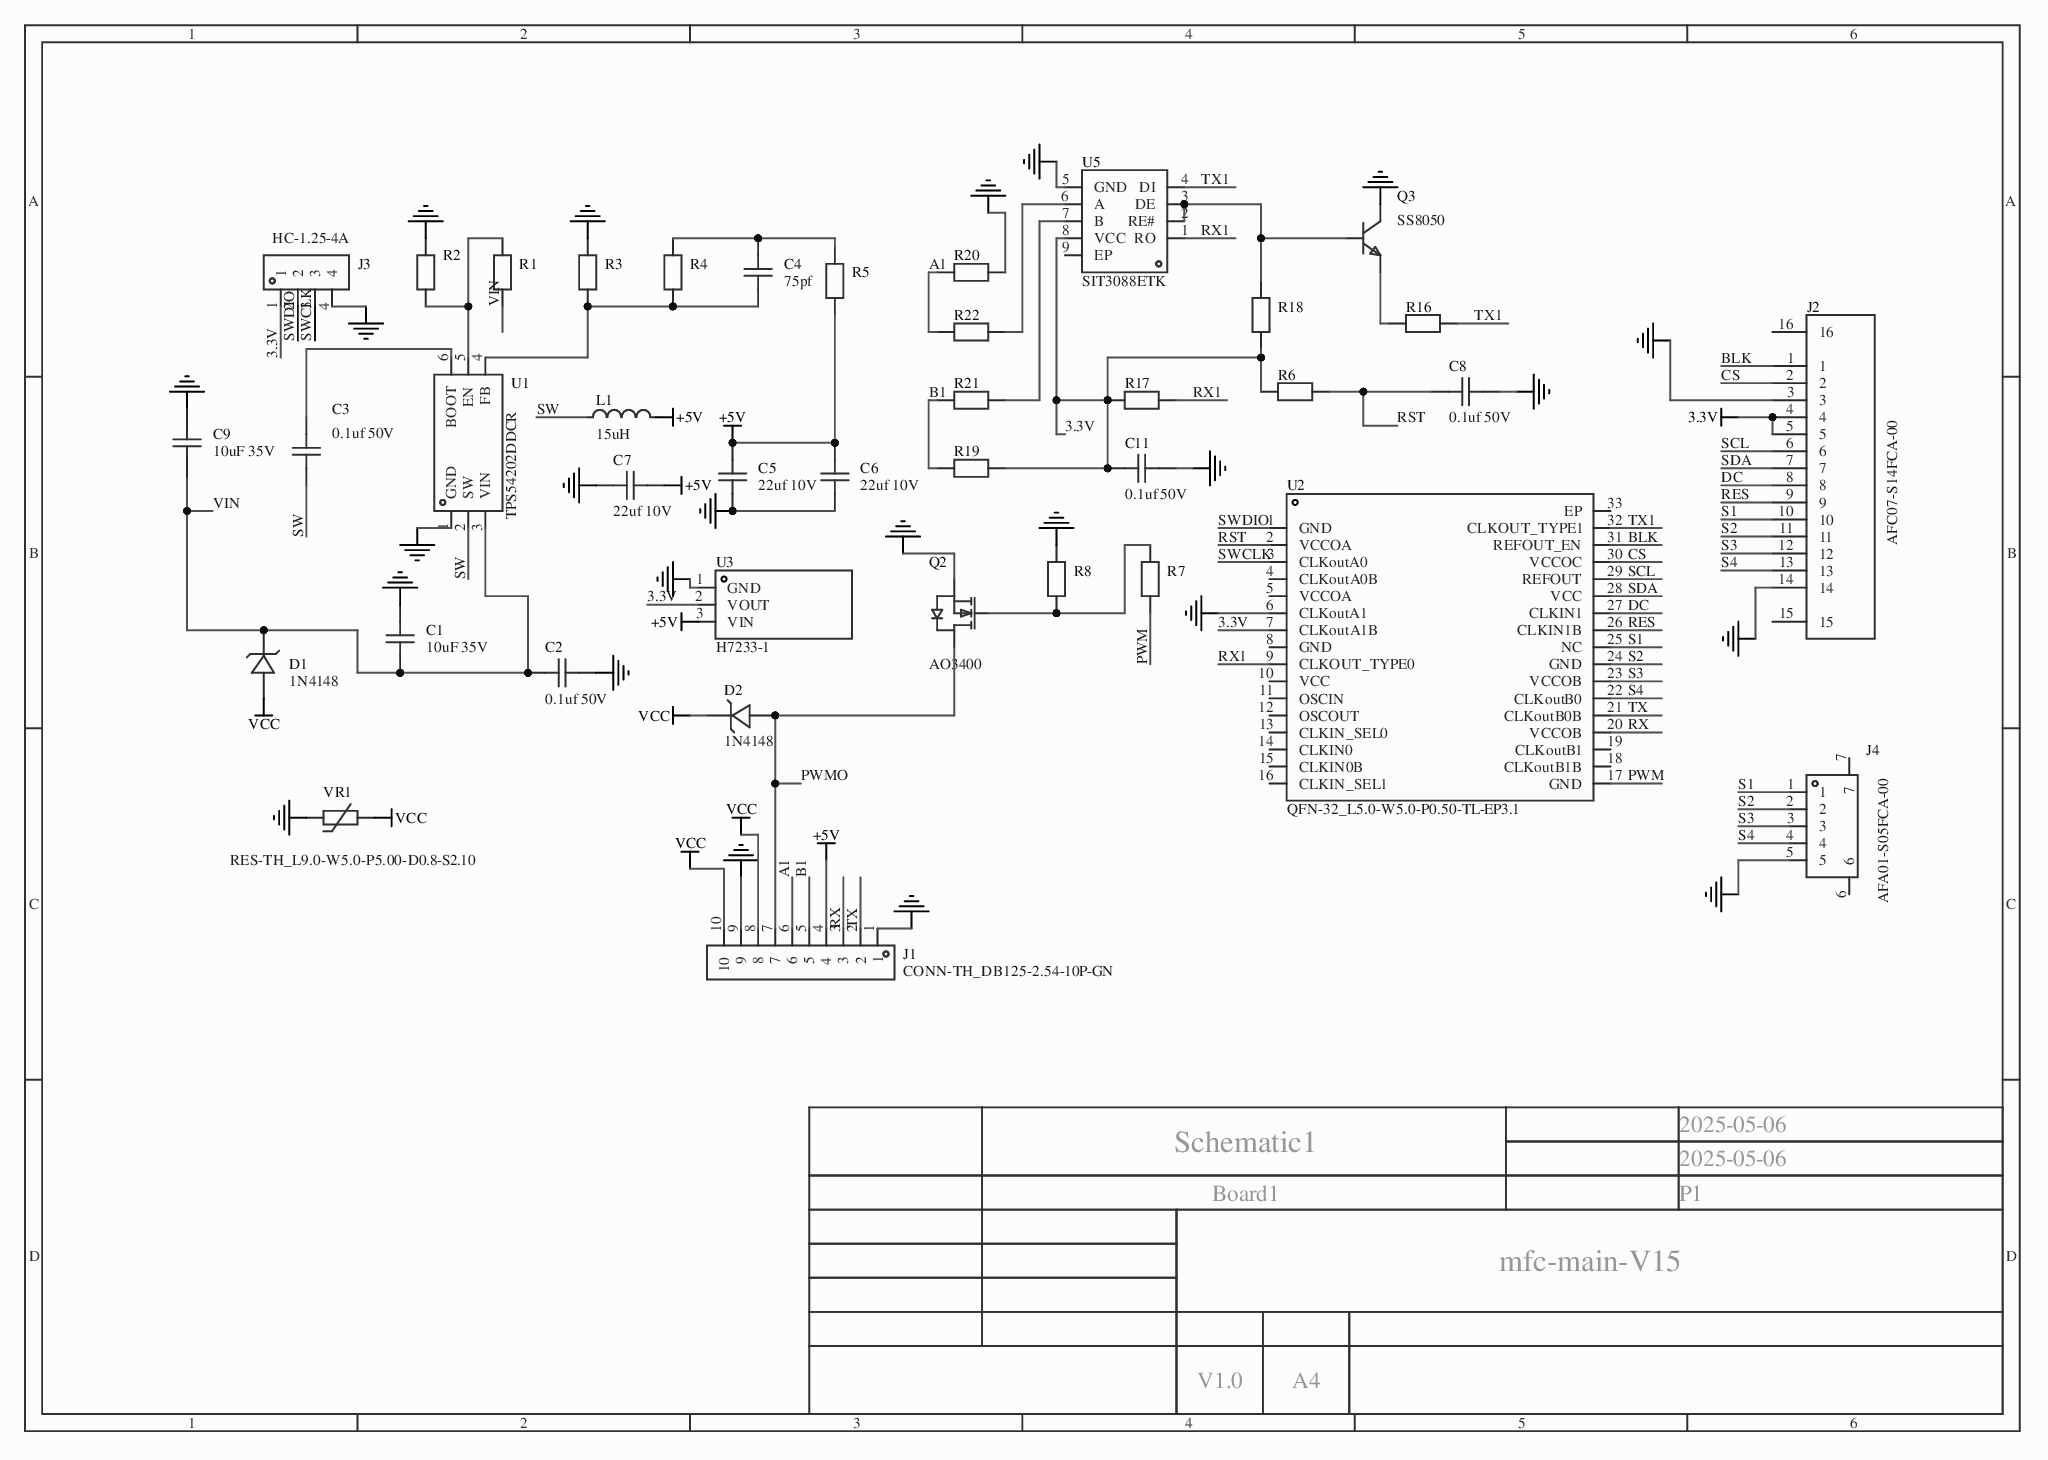
[diagram p0: MISC84392-2.SchDoc]
# Altium project MISC84392-4.PrjPcb
1 sheet, 39 parts. Net scope: global (net labels, ports and power ports of the same name join across sheets).
Board file: MISC84392.PcbDoc

## Sheet MISC84392-2.SchDoc
size 307 x 218 mm; Symbol: Drawing-Symbol_A4; Device: Drawing-Symbol_A4; Version: V1.0; Page Size: A4; @Project Name: mfc-main-V15; @Page Count: 1; @Update Date: 2025-05-06; @Create Date: 2025-05-06; @Schematic Name: Schematic1; @Page No: 1; @Page Name: P1; @Create Time: 07:06:31; @Update Time: 15:06:31; Width: 1170; Height: 825; Region Start: 1; X Region Count: 6; Y Region Count: 4; Blade Width: 10; Title Block Position: 3; @Board Name: Board1

### Parts
C1  10uF 35V  [C0805]
C2  0.1uf 50V  [C0603]
C3  0.1uf 50V  [C0603]
C4  75pf  [C0603]
C5  22uf 10V  [C0603]
C6  22uf 10V  [C0603]
C7  22uf 10V  [C0603]
C8  0.1uf 50V  [C0603]
C9  10uF 35V  [C0805]
C11  0.1uf 50V  [C0603]
D1  1N4148  [SOD-123_L2.7-W1.7-LS3.8-RD]
D2  1N4148  [SOD-123_L2.7-W1.7-LS3.8-RD]
J1  CONN-TH_DB125-2.54-10P-GN  [CONN-TH_DB125-2.54-10P-GN]
J2  AFC07-S14FCA-00  [FPC-SMD_14P-P0.50_AFC07-S14FCA-00]
J3  HC-1.25-4A  [CONN-TH_4P-P1.25_HCTL_HC-1.25-4A]
J4  AFA01-S05FCA-00  [FPC-SMD_AFA01-S05FCA-00]
L1  15uH  [IND-SMD_L3.5-W3.0]
Q2  AO3400  [SOT-23-3_L2.9-W1.3-P1.90-LS2.4-BL-2]
Q3  SS8050  [SOT-23-3_L2.9-W1.3-P1.90-LS2.4-BR]
R1  (no value)  [R0603]
R2  (no value)  [R0603]
R3  (no value)  [R0603]
R4  (no value)  [R0603]
R5  (no value)  [R0603]
R6  (no value)  [R0603]
R7  (no value)  [R0603]
R8  (no value)  [R0603]
R16  (no value)  [R0603]
R17  (no value)  [R0603]
R18  (no value)  [R0603]
R19  (no value)  [R0603]
R20  (no value)  [R0603]
R21  (no value)  [R0603]
R22  (no value)  [R0603]
U1  TPS54202DDCR  [SOT-23-6_L2.9-W1.6-P0.95-LS2.8-BL]
U2  QFN-32_L5.0-W5.0-P0.50-TL-EP3.1  [QFN-32_L5.0-W5.0-P0.50-TL-EP3.1]
U3  H7233-1  [SOT-23-3_L2.9-W1.3-P1.90-LS2.4-BR]
U5  SIT3088ETK  [DFN-8_L3.0-W3.0-P0.65-BL-EP]
VR1  RES-TH_L9.0-W5.0-P5.00-D0.8-S2.10  [RES-TH_L9.0-W5.0-P5.00-D0.8-S2.10]

### Nets
3.3V: C11.2 J2.4 J2.5 J3.1 R6.1 R17.1 R18.1 R19.2 U2.7(CLKoutA1B) U3.2(VOUT) U5.8(VCC)
+5V: C5.1 C6.1 C7.1 J1.4 L1.2 R5.1 U3.3(VIN)
GND: C1.2 C2.1 C5.2 C6.2 C7.2 C8.1 C9.2 C11.1 J1.1 J1.9 J2.3 J2.14 J3.4 J4.5 Q2.2(S) Q3.3(C) R2.2 R3.2 R8.2 R20.2 U1.1(GND) U2.6(CLKoutA1) U3.1(GND) U5.5(GND) VR1.1
VCC: D1.2(A) D2.1(K) J1.8 J1.10 VR1.2
A1: J1.6 R20.1 R22.1
B1: J1.5 R19.1 R21.1
BLK: J2.1 U2.31(REFOUT_EN)
CS: J2.2 U2.30(VCCOC)
DC: J2.8 U2.27(CLKIN1)
PWM: R7.1 U2.17(GND)
PWMO: D2.2(A) J1.7 Q2.3(D)
RES: J2.9 U2.26(CLKIN1B)
RST: C8.2 R6.2 U2.2(VCCOA)
RX: J1.3 U2.20(VCCOB)
RX1: R17.2 U2.9(CLKOUT_TYPE0) U5.1(RO)
S1: J2.10 J4.1 U2.25(NC)
S2: J2.11 J4.2 U2.24(GND)
S3: J2.12 J4.3 U2.23(VCCOB)
S4: J2.13 J4.4 U2.22(CLKoutB0)
SCL: J2.6 U2.29(REFOUT)
SDA: J2.7 U2.28(VCC)
SW: C3.1 L1.1 U1.2(SW)
SWCLK: J3.3 U2.3(CLKoutA0)
SWDIO: J3.2 U2.1(GND)
TX: J1.2 U2.21(CLKoutB0B)
TX1: R16.2 U2.32(CLKOUT_TYPE1) U5.4(DI)
VIN: C1.1 C2.2 C9.1 D1.1(K) R1.1 U1.3(VIN)
NetC3_2: C3.2 U1.6(BOOT)
NetC4_1: C4.1 R4.2 R5.2
NetC4_2: C4.2 R3.1 R4.1 U1.4(FB)
NetQ2_1: Q2.1(G) R7.2 R8.1
NetQ3_1: Q3.1(B) R18.2 U5.2(RE#) U5.3(DE)
NetQ3_2: Q3.2(E) R16.1
NetR1_2: R1.2 R2.1 U1.5(EN)
NetR21_2: R21.2 U5.7(B)
NetR22_2: R22.2 U5.6(A)

Not connected (* = marked no-connect by the designer): J2 15 16; J4 6 7; U2 4(CLKoutA0B) 5(VCCOA) 8(GND) 10(VCC) 11(OSCIN) 12(OSCOUT) 13(CLKIN_SEL0) 14(CLKIN0) 15(CLKIN0B) 16(CLKIN_SEL1) 18(CLKoutB1B) 19(CLKoutB1) 33(EP); U5 9(EP)

### Notes on the sheet
- 1
- 2
- 3
- 4
- 5
- 6
- A
- B
- C
- Schematic1
- 2025-05-06
- Board1
- P1
- D
- mfc-main-V15
- V1.0
- A4

### Library data of the parts
C1 C9 = CL21A106KAYNNNE_C15850: Add into BOM: yes; Voltage Rated: 25V; Temperature Coefficient: X5R; Symbol: CL21A106KAYNNNE; Device: CL21A106KAYNNNE_C15850; Manufacturer Part: CL21A106KAYNNNE; Supplier Footprint: 0805; Datasheet: https://atta.szlcsc.com/upload/public/pdf/source/20160218/1457707763339.pdf; Supplier: LCSC; Convert to PCB: yes; Value: 10uF 35V
C2-C8 C11 = CT41-0603-2F4-50V-0.1uF-M(N): Add into BOM: yes; Symbol: CT41-0603-2F4-50V-0.1UF-M(N); Device: CT41-0603-2F4-50V-0.1uF-M(N); Supplier Part: C138344; Manufacturer Part: CT41-0603-2F4-50V-0.1uF-M(N); Supplier Footprint: 0603; Supplier: LCSC; Convert to PCB: yes
D1 D2 = 1N4148: Symbol: 1N4148_C9900009645; Add into BOM: yes; Device: 1N4148; LCSC Part Name: 1N4148; Supplier Part: C9900009645; Manufacturer Part: 1N4148; Supplier Footprint: SOD-123_L2.7-W1.7--LS3.8-RD; Supplier: LCSC; Convert to PCB: yes
J1 = DB125-2.54-10P-GN-S: Add into BOM: yes; Number of Positions or Pins: 1x10P; Pitch: 2.54mm; Number of PINs Per Row: 10; Current Rating: 7A; Voltage Rating (Max): 150V; Wire Gauge - AWG: 18~26; Wire Gauge - mm2: 1; Symbol: DB125-2.54-10P-GN; Device: DB125-2.54-10P-GN-S; Supplier Part: C918128; Manufacturer Part: DB125-2.54-10P-GN-S; Datasheet: https://atta.szlcsc.com/upload/public/pdf/source/20230106/BCD3A0BE1EB95DC3E813F1745F022035.pdf; Supplier: LCSC; Convert to PCB: yes; Number of Pins: 10P; Number of Rows: 1
J2 = AFC07-S14FCA-00: Add into BOM: yes; Number of Contacts: 14P; Pitch: 0.5mm; FFC, FCB Thickness: 0.3mm; Symbol: AFC07-S14FCA-00; Device: AFC07-S14FCA-00; Supplier Part: C262561; Manufacturer Part: AFC07-S14FCA-00; Datasheet: https://atta.szlcsc.com/upload/public/pdf/source/20190726/C11047_78689421E6D6672DE8D11ECCF89B3729.pdf; Supplier: LCSC; Convert to PCB: yes; Height Above Board: 2mm
J3 = HC-1.25-4A: Add into BOM: yes; Pins Structure: 1x4P; Pitch: 1.25mm; Reference Series: PicoBlade(MX 1.25); Number of PINs Per Row: 4; Current Rating (Max): 1A; Rated Voltage (Max): 125V; Plastic Material: PA46; Flame Retardant Rating: UL94V-0; Z-Height of the Board: 4.7mm; X-Length of Bottom Edge on Board (Spacing Line): 6.75mm; Y-Width of Bottom Edge on Board: 3.2mm; Symbol: HC-1.25-4A; Device: HC-1.25-4A; Supplier Part: C2845522; Manufacturer Part: HC-1.25-4A; Datasheet: https://atta.szlcsc.com/upload/public/pdf/source/20230707/9C9BC153C15CECDA5FD17EC6041C1792.pdf; Supplier: LCSC; Convert to PCB: yes; Number of Pins: 4P; Number of Rows: 1; Row Spacing: -; Supplementary Features: -; Colour: -
J4 = AFA01-S05FCA-00: Add into BOM: yes; Number of Contacts: 5P; Pitch: 1mm; FFC, FCB Thickness: 0.3mm; Symbol: AFA01-S05FCA-00; Device: AFA01-S05FCA-00; Supplier Part: C262753; Manufacturer Part: AFA01-S05FCA-00; Datasheet: https://atta.szlcsc.com/upload/public/pdf/source/20210330/C262753_4BD8204516538AD75814ADC10978F9F3.pdf; Supplier: LCSC; Convert to PCB: yes; Height Above Board: 2mm
L1 = CMLF0302-150MTT: Add into BOM: yes; Rated Current: 950mA; Symbol: CMLF0302-150MTT; Device: CMLF0302-150MTT; Supplier Part: C405096; Manufacturer Part: CMLF0302-150MTT; Supplier Footprint: SMD,3.5x3mm; Datasheet: https://atta.szlcsc.com/upload/public/pdf/source/20190722/C405106_79BE834BCBEB8E6D15D29C738CB0B805.pdf; Supplier: LCSC; Convert to PCB: yes; Value: 15uH
Q2 = AO3400: Symbol: AO3400_C9900013365; Add into BOM: yes; Device: AO3400; LCSC Part Name: AO3400; Supplier Part: C9900013365; Manufacturer Part: AO3400; Supplier Footprint: SOT-23; Supplier: LCSC; Convert to PCB: yes
Q3 = SS8050: Symbol: SS8050_C2931717; Add into BOM: yes; Device: SS8050; LCSC Part Name: NPN 25V 1.5A 120-400 SOT-23; Supplier Part: C2931717; Manufacturer Part: SS8050; Supplier Footprint: SOT-23; Datasheet: https://atta.szlcsc.com/upload/public/pdf/source/20220106/99F9A3DFCBDD91265C711555CE6390BF.pdf; Supplier: LCSC; Convert to PCB: yes
R1-R8 R16-R22 = RT0603BRD07105KL: Add into BOM: yes; Power(Watts): 100mW; Symbol: RT0603BRD07105KL; Device: RT0603BRD07105KL; Manufacturer Part: RT0603BRD07105KL; Supplier Footprint: 0603; Datasheet: https://atta.szlcsc.com/upload/public/pdf/source/20200610/C326738_5639A9F1B6EB6E4AE2197577D3456E7F.pdf; Supplier: LCSC; Convert to PCB: yes
  R2: Supplier Part: C861072
U1 = TPS54202DDCR: Add into BOM: yes; Input Voltage: 4.5V~28V; Output Current: 2A; Switching Frequency: 500kHz; Number of Outputs: 1; Quiescent Current (Iq): 45uA; Symbol: TPS54202DDCR; Device: TPS54202DDCR; Supplier Part: C191884; Manufacturer Part: TPS54202DDCR; Supplier Footprint: SOT-23-6; Datasheet: https://www.ti.com/cn/lit/gpn/tps54202; Supplier: LCSC; Convert to PCB: yes; Output Voltage: -
U2 = NCS25D34: Add into BOM: yes; Symbol: NCS25D34; Device: NCS25D34; LCSC Part Name: NCS25D34; Supplier Part: C9900091701; Manufacturer Part: NCS25D34; Supplier Footprint: QFN-32_L5.0-W5.0-P0.50-TL-EP3.1; Supplier: LCSC; Convert to PCB: yes
U3 = H7233-1: Symbol: H7233-1_C277859; Add into BOM: yes; Voltage - Supply: 15V; Output Voltage: 3.3V; Output Current: 400mA; Power Supply Rejection Ratio (PSRR): 40dB@(1kHz); Voltage Dropout: 850mV@(500mA); Number of Outputs: 1; Device: H7233-1; Supplier Part: C277859; Manufacturer Part: H7233-1; Supplier Footprint: SOT-23-3; Datasheet: https://atta.szlcsc.com/upload/public/pdf/source/20180913/C277861_5081AFEFA5E5EDF8F706F1E9069AF901.pdf; Supplier: LCSC; Convert to PCB: yes
U5 = SIT3088ETK: Add into BOM: yes; Number of Driver: 1; Supply Voltage: 3V~5.5V; Data Rate: 14Mbps; Node Number: 256; Symbol: SIT3088ETK; Device: SIT3088ETK; Supplier Part: C601076; Manufacturer Part: SIT3088ETK; Supplier Footprint: DFN-8-EP(3x3); Datasheet: https://atta.szlcsc.com/upload/public/pdf/source/20200610/C601074_2E843880C44A2DA1B7E0D38765D8E5FA.pdf; Supplier: LCSC; Convert to PCB: yes; Number of receiver: 1
VR1 = FTR07D390K: Add into BOM: yes; Varistor Voltage: 35V~43V; Clamping Voltage: 77V; Allowable Voltage (DC): 31V; Allowable Voltage (AC): 25V; Peak Current: 250A; Maximum Energy: 2.1J; Symbol: FTR07D390K; Device: FTR07D390K; Supplier Part: C693447; Manufacturer Part: FTR07D390K; Datasheet: https://atta.szlcsc.com/upload/public/pdf/source/20200716/C693448_B319437BF9A7FC54F7E4F3EEAC321399.pdf; Supplier: LCSC; Convert to PCB: yes; Typical Capatitance: -